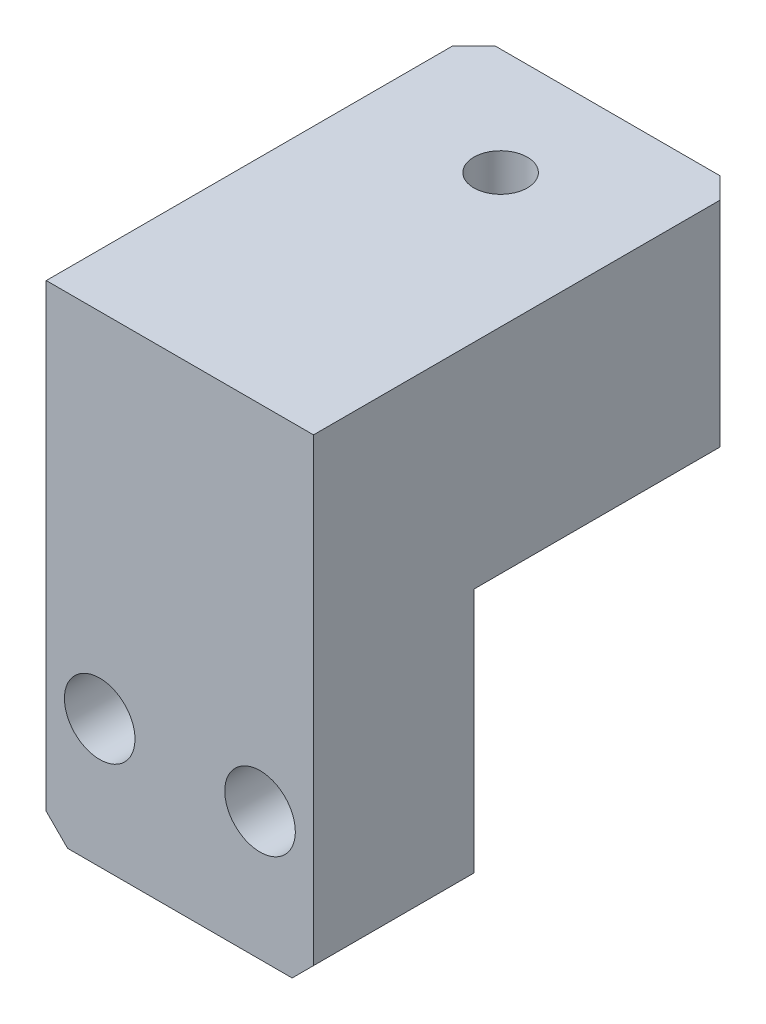
SolidWorks part; units mm, degrees
ref_plane "前视基准面" through (0, 0, 0) normal (0, 0, 1) x (1, 0, 0)
ref_plane "上视基准面" through (0, 0, 0) normal (0, 1, 0) x (1, 0, 0)
ref_plane "右视基准面" through (0, 0, 0) normal (1, 0, 0) x (0, 0, -1)
sketch "草图1" plane through (0, 0, 0) normal (0, 1, 0) x (1, 0, 0)
  line L1 (0, 0) -> (25, 0)
  line L2 (0, 0) -> (0, 40)
  line L3 (0, 40) -> (25, 40)
  line L4 (25, 0) -> (25, 40)
  dimension "D1" = 40
  dimension "D2" = 25
extrude "凸台-拉伸1" add sketch "草图1" along normal blind 20
chamfer "倒角1" distance 2 angle 45 2 edges at (0, 10, -40) (25, 10, -40)
sketch "草图5" plane through (0, 0, 0) normal (0, -1, 0) x (-1, 0, 0)
  line L0 (0, 0) -> (-25, 0) construction
  line L1 (-23, 40) -> (-2, 40) construction
  point P0 (-12.5, 30)
  point P5 (-12.5, 0)
  dimension "D1" = 10
hole_wizard "M6 螺纹孔1" positions "草图5" profile "草图4" tap size "M6" standard "GB" end condition through all
sketch "草图4" plane through (12.5, 0, -30) normal (1, 0, 0) x (0, 0, -1)
  line L0 (0, 0) -> (0, 20)
  line L1 (0, 20) -> (2.5, 20)
  line L2 (2.5, 20) -> (2.5, 0)
  line L5 (2.5, 0) -> (0, 0)
  line L11 (0, -6.35) -> (0, 107.95) construction
  dimension "通孔螺纹孔钻头直径" = 5
  dimension "通孔螺纹孔钻头深度" = 20
cosmetic thread "孔螺纹线1" parameters "D2"=6
sketch "草图6" plane through (25, 0, 0) normal (1, 0, 0) x (0, 0, -1)
  line L1 (0, 0) -> (15, 0)
  line L2 (0, 0) -> (0, -25)
  line L3 (0, -25) -> (15, -25)
  line L4 (15, 0) -> (15, -25)
  dimension "D1" = 15
  dimension "D2" = 25
extrude "凸台-拉伸2" add sketch "草图6" against normal up to surface (25 mm away) up to face at (0, 10, -19)
sketch "草图9" plane through (0, 0, -15) normal (0, 0, -1) x (-1, 0, 0)
  line L0 (-12.5, 0) -> (-12.5, -32.7269) construction
  line L1 (0, 0) -> (-25, 0) construction
  line L3 (0, -25) -> (-25, -25) construction
  point P0 (-20, -13)
  point P2 (-5, -13)
  dimension "D1" = 15
  dimension "D2" = 12
hole_wizard "M6 间隙孔1" positions "草图9" profile "草图8" hole size "M6" standard "GB" end condition through all
sketch "草图8" plane through (20, -13, -15) normal (1, 0, 0) x (0, 1, 0)
  line L0 (0, 0) -> (0, 15)
  line L1 (0, 15) -> (3.3, 15)
  line L2 (3.3, 15) -> (3.3, 0)
  line L5 (3.3, 0) -> (0, 0)
  line L11 (0, -6.35) -> (0, 107.95) construction
  dimension "通孔孔直径" = 6.6
  dimension "通孔孔深度" = 15
chamfer "倒角2" distance 2 angle 45 2 edges at (0, -25, -7.5) (25, -25, -7.5)
